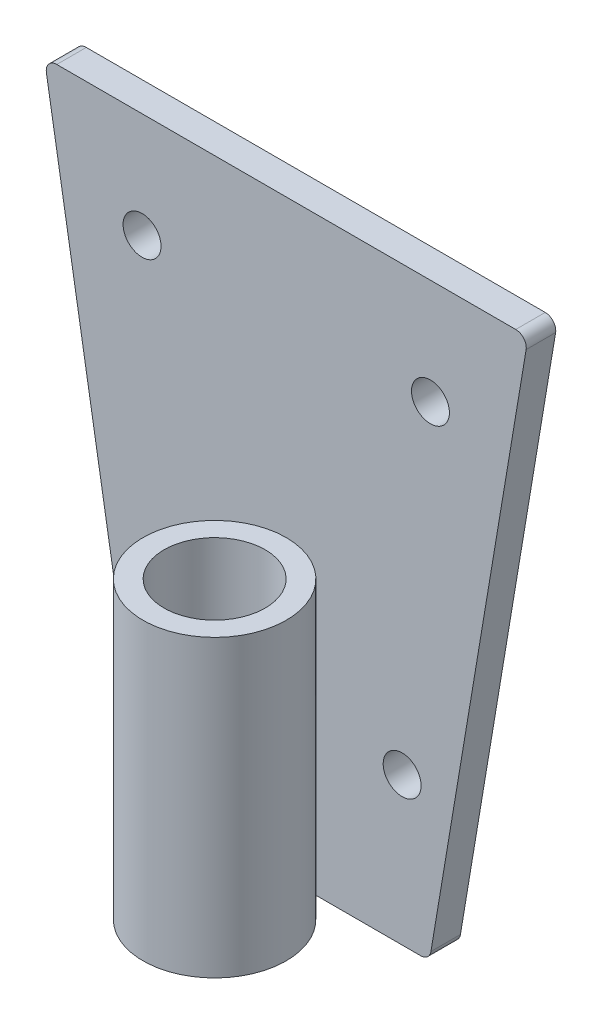
SolidWorks part; units mm, degrees
material "普通碳钢"
ref_plane "前视基准面" through (0, 0, 0) normal (0, 0, 1) x (1, 0, 0)
ref_plane "上视基准面" through (0, 0, 0) normal (0, 1, 0) x (1, 0, 0)
ref_plane "右视基准面" through (0, 0, 0) normal (1, 0, 0) x (0, 0, -1)
sketch "草图1" plane through (0, 0, 0) normal (0, 0, 1) x (1, 0, 0)
  line L0 (-67.969, -2335) -> (67.969, -2335)
  line L1 (67.969, -2335) -> (114.8249, -2055)
  line L2 (67.969, -2335) -> (446.835, -70.9863) construction
  line L3 (114.8249, -2055) -> (-114.8249, -2055)
  line L4 (-67.969, -2335) -> (-446.835, -70.9863) construction
  line L5 (-114.8249, -2055) -> (-67.969, -2335)
  dimension "D1" = 280
extrude "凸台-拉伸1" add sketch "草图1" along normal blind 14
sketch "草图2" plane through (0, -2335, 0) normal (0, -1, 0) x (1, 0, 0)
  line L0 (-67.969, 14) -> (67.969, 14) construction
  circle A0 centre (0, 48) radius 34
  circle A1 centre (0, 48) radius 24
  dimension "D1" = 68
  dimension "D2" = 48
extrude "凸台-拉伸2" add sketch "草图2" against normal blind 140 separate body
fillet "圆角1" radius 5 4 edges at (-114.8249, -2055, 7) (114.8249, -2055, 7) (-67.969, -2335, 7) (67.969, -2335, 7)
hole_wizard "Ø18.0 (18) 直径孔1" positions "草图4" profile "草图5" hole size "Ø18.0" standard "ISO"
sketch "草图4" plane through (0, 0, 0) normal (0, 0, -1) x (-1, 0, 0)
  point P0 (-68.4373, -2105)
  point P3 (-55, -2265)
  point P6 (55, -2265)
  point P9 (68.4373, -2105)
sketch "草图5" plane through (68.4373, -2105, 0) normal (1, 0, 0) x (0, 1, 0)
  line L0 (0, 0) -> (0, 65.4077)
  line L1 (0, 65.4077) -> (9, 60)
  line L2 (9, 60) -> (9, 0)
  line L5 (9, 0) -> (0, 0)
  line L10 (0, 65.4077) -> (-9, 60) construction
  line L11 (0, -6.35) -> (0, 107.95) construction
  dimension "孔直径" = 18
  dimension "孔深度" = 60
  dimension "导头角度" = 118
